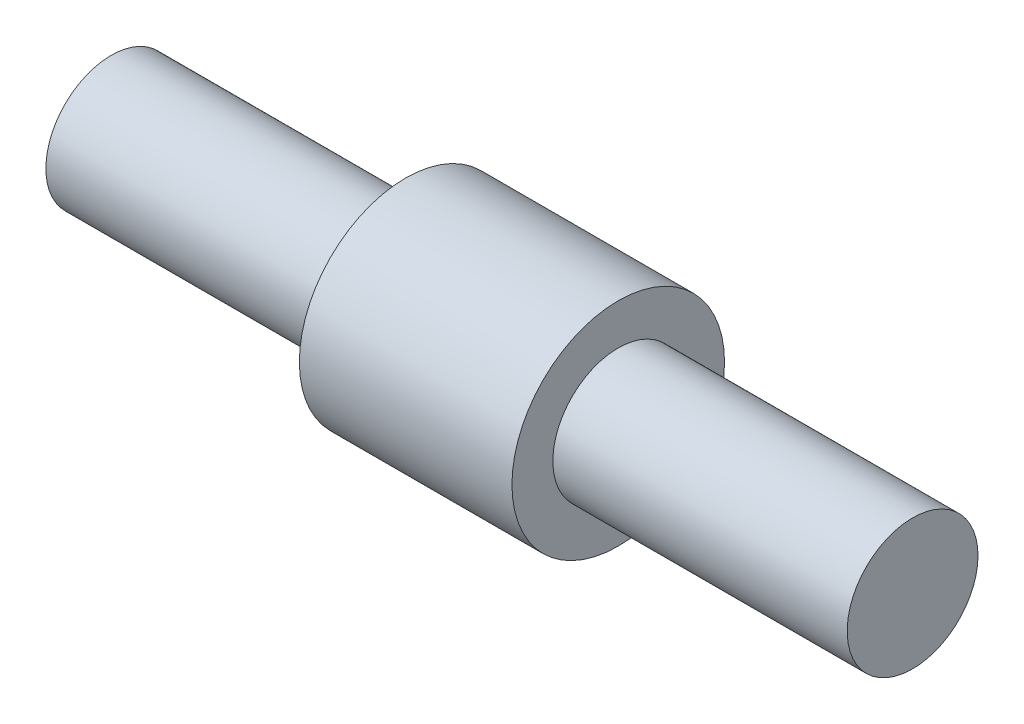
SolidWorks part; units mm, degrees
material "AISI 1045 Steel, cold drawn"
ref_plane "Front Plane" through (0, 0, 0) normal (0, 0, 1) x (1, 0, 0)
ref_plane "Top Plane" through (0, 0, 0) normal (0, 1, 0) x (1, 0, 0)
ref_plane "Right Plane" through (0, 0, 0) normal (1, 0, 0) x (0, 0, -1)
sketch "Sketch1" plane through (0, 0, 0) normal (1, 0, 0) x (0, 0, -1)
  circle A0 centre (0, 0) radius 6.5
  dimension "D1" = 13
extrude "Boss-Extrude1" add sketch "Sketch1" along normal mid plane 13
sketch "Sketch3" plane through (6.5, 0, 0) normal (1, 0, 0) x (0, 0, -1)
  circle A0 centre (0, 0) radius 4
  dimension "D1" = 8
extrude "Boss-Extrude2" add sketch "Sketch3" along normal blind 18
mirror "Mirror1" about plane through (0, 0, 0) normal (1, 0, 0) of "Boss-Extrude2"
